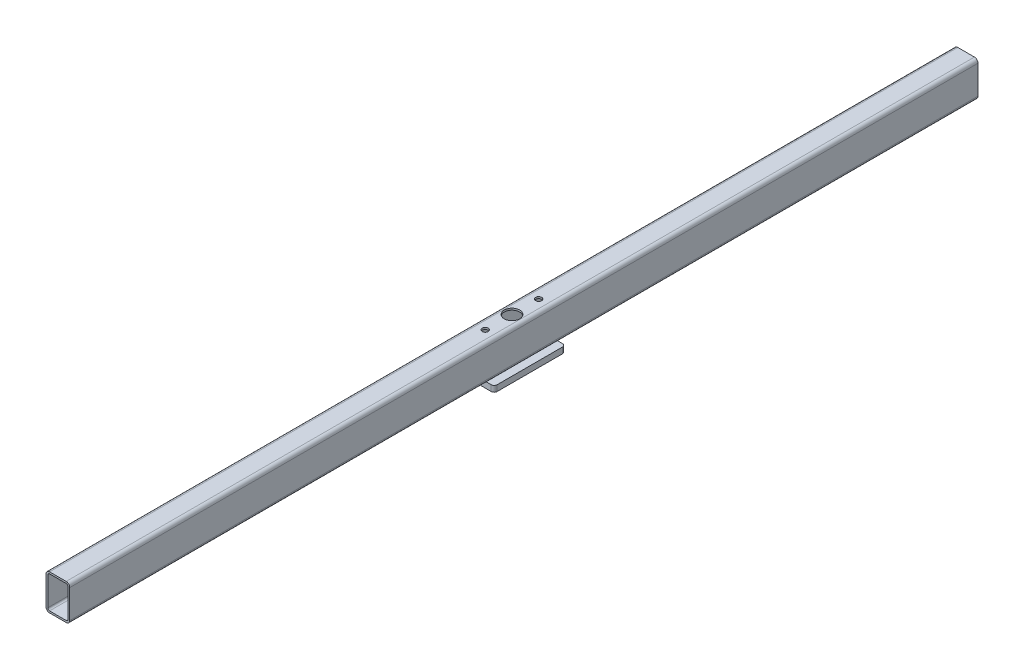
from build123d import *

# Parameters (mm, degrees)
GB_6728_1986_RECTANGULAR_HOLLOW_SECTION_DEPTH = 1530
SKETCH5_R                                     = 13
CUT_EXTRUDE1_DEPTH                            = 214
SKETCH6_W                                     = 60
SKETCH6_H                                     = 120
SKETCH6_R                                     = 13
BOSS_EXTRUDE1_DEPTH                           = 10
SKETCH7_R                                     = 5
CUT_EXTRUDE2_DEPTH                            = 1532.469882172
FILLET1_R                                     = 5


with BuildPart() as part:
    # Sketch14 → Gb/6728-1986 rectangular hollow section 060 X 40 X 3 (new body)
    with BuildSketch(Plane(origin=(0, 0, 0), x_dir=(-1, 0, 0), z_dir=(0, 0, -1))):
        with BuildLine():
            Line((-14, -30), (14, -30))
            ThreePointArc((14, -30), (18.242640687, -28.242640687), (20, -24))
            Line((20, -24), (20, 24))
            ThreePointArc((20, 24), (18.242640687, 28.242640687), (14, 30))
            Line((14, 30), (-14, 30))
            ThreePointArc((-14, 30), (-18.242640687, 28.242640687), (-20, 24))
            Line((-20, 24), (-20, -24))
            ThreePointArc((-20, -24), (-18.242640687, -28.242640687), (-14, -30))
        make_face()
        with BuildLine():
            Line((-14, -27), (14, -27))
            ThreePointArc((14, -27), (16.121320344, -26.121320344), (17, -24))
            Line((17, -24), (17, 24))
            ThreePointArc((17, 24), (16.121320344, 26.121320344), (14, 27))
            Line((14, 27), (-14, 27))
            ThreePointArc((-14, 27), (-16.121320344, 26.121320344), (-17, 24))
            Line((-17, 24), (-17, -24))
            ThreePointArc((-17, -24), (-16.121320344, -26.121320344), (-14, -27))
        make_face(mode=Mode.SUBTRACT)
    extrude(amount=GB_6728_1986_RECTANGULAR_HOLLOW_SECTION_DEPTH)

    # Sketch5 → Cut-Extrude1 (cut)
    with BuildSketch(Plane(origin=(0, 30, 0), x_dir=(1, 0, 0), z_dir=(0, 1, 0))):
        with Locations(Location((0, 765, 0), (0, 0, 270))):
            Circle(SKETCH5_R)
    extrude(amount=-CUT_EXTRUDE1_DEPTH, mode=Mode.SUBTRACT)

    # Sketch7 → Cut-Extrude2 (cut, through all)
    with BuildSketch(Plane.XZ.offset(30)):
        with Locations(Location((0, -720, 0), (0, 0, 270))):
            Circle(SKETCH7_R)
        with Locations(Location((0, -810, 0), (0, 0, 270))):
            Circle(SKETCH7_R)
    extrude(amount=-CUT_EXTRUDE2_DEPTH, mode=Mode.SUBTRACT)


with BuildPart() as body_2:
    # Sketch6 → Boss-Extrude1 (new body)
    with BuildSketch(Plane.XZ.offset(30)):
        with Locations((0, -765)):
            Rectangle(SKETCH6_W, SKETCH6_H)
        with Locations(Location((0, -765, 0), (0, 0, 270))):
            Circle(SKETCH6_R, mode=Mode.SUBTRACT)
        with BuildLine():
            Line((4.5, -715), (4.5, -725))
            ThreePointArc((4.5, -725), (0, -729.5), (-4.5, -725))
            Line((-4.5, -725), (-4.5, -715))
            ThreePointArc((-4.5, -715), (0, -710.5), (4.5, -715))
        make_face(mode=Mode.SUBTRACT)
        with BuildLine():
            Line((4.5, -805), (4.5, -815))
            ThreePointArc((4.5, -815), (0, -819.5), (-4.5, -815))
            Line((-4.5, -815), (-4.5, -805))
            ThreePointArc((-4.5, -805), (0, -800.5), (4.5, -805))
        make_face(mode=Mode.SUBTRACT)
    extrude(amount=BOSS_EXTRUDE1_DEPTH)

    # Fillet1
    fillet1_edges = [body_2.edges().sort_by_distance(p)[0] for p in [
        (30, -35, -825),
        (-30, -35, -825),
        (-30, -35, -705),
        (30, -35, -705),
    ]]
    fillet(fillet1_edges, radius=FILLET1_R)


solid = Compound([part.part, body_2.part])
